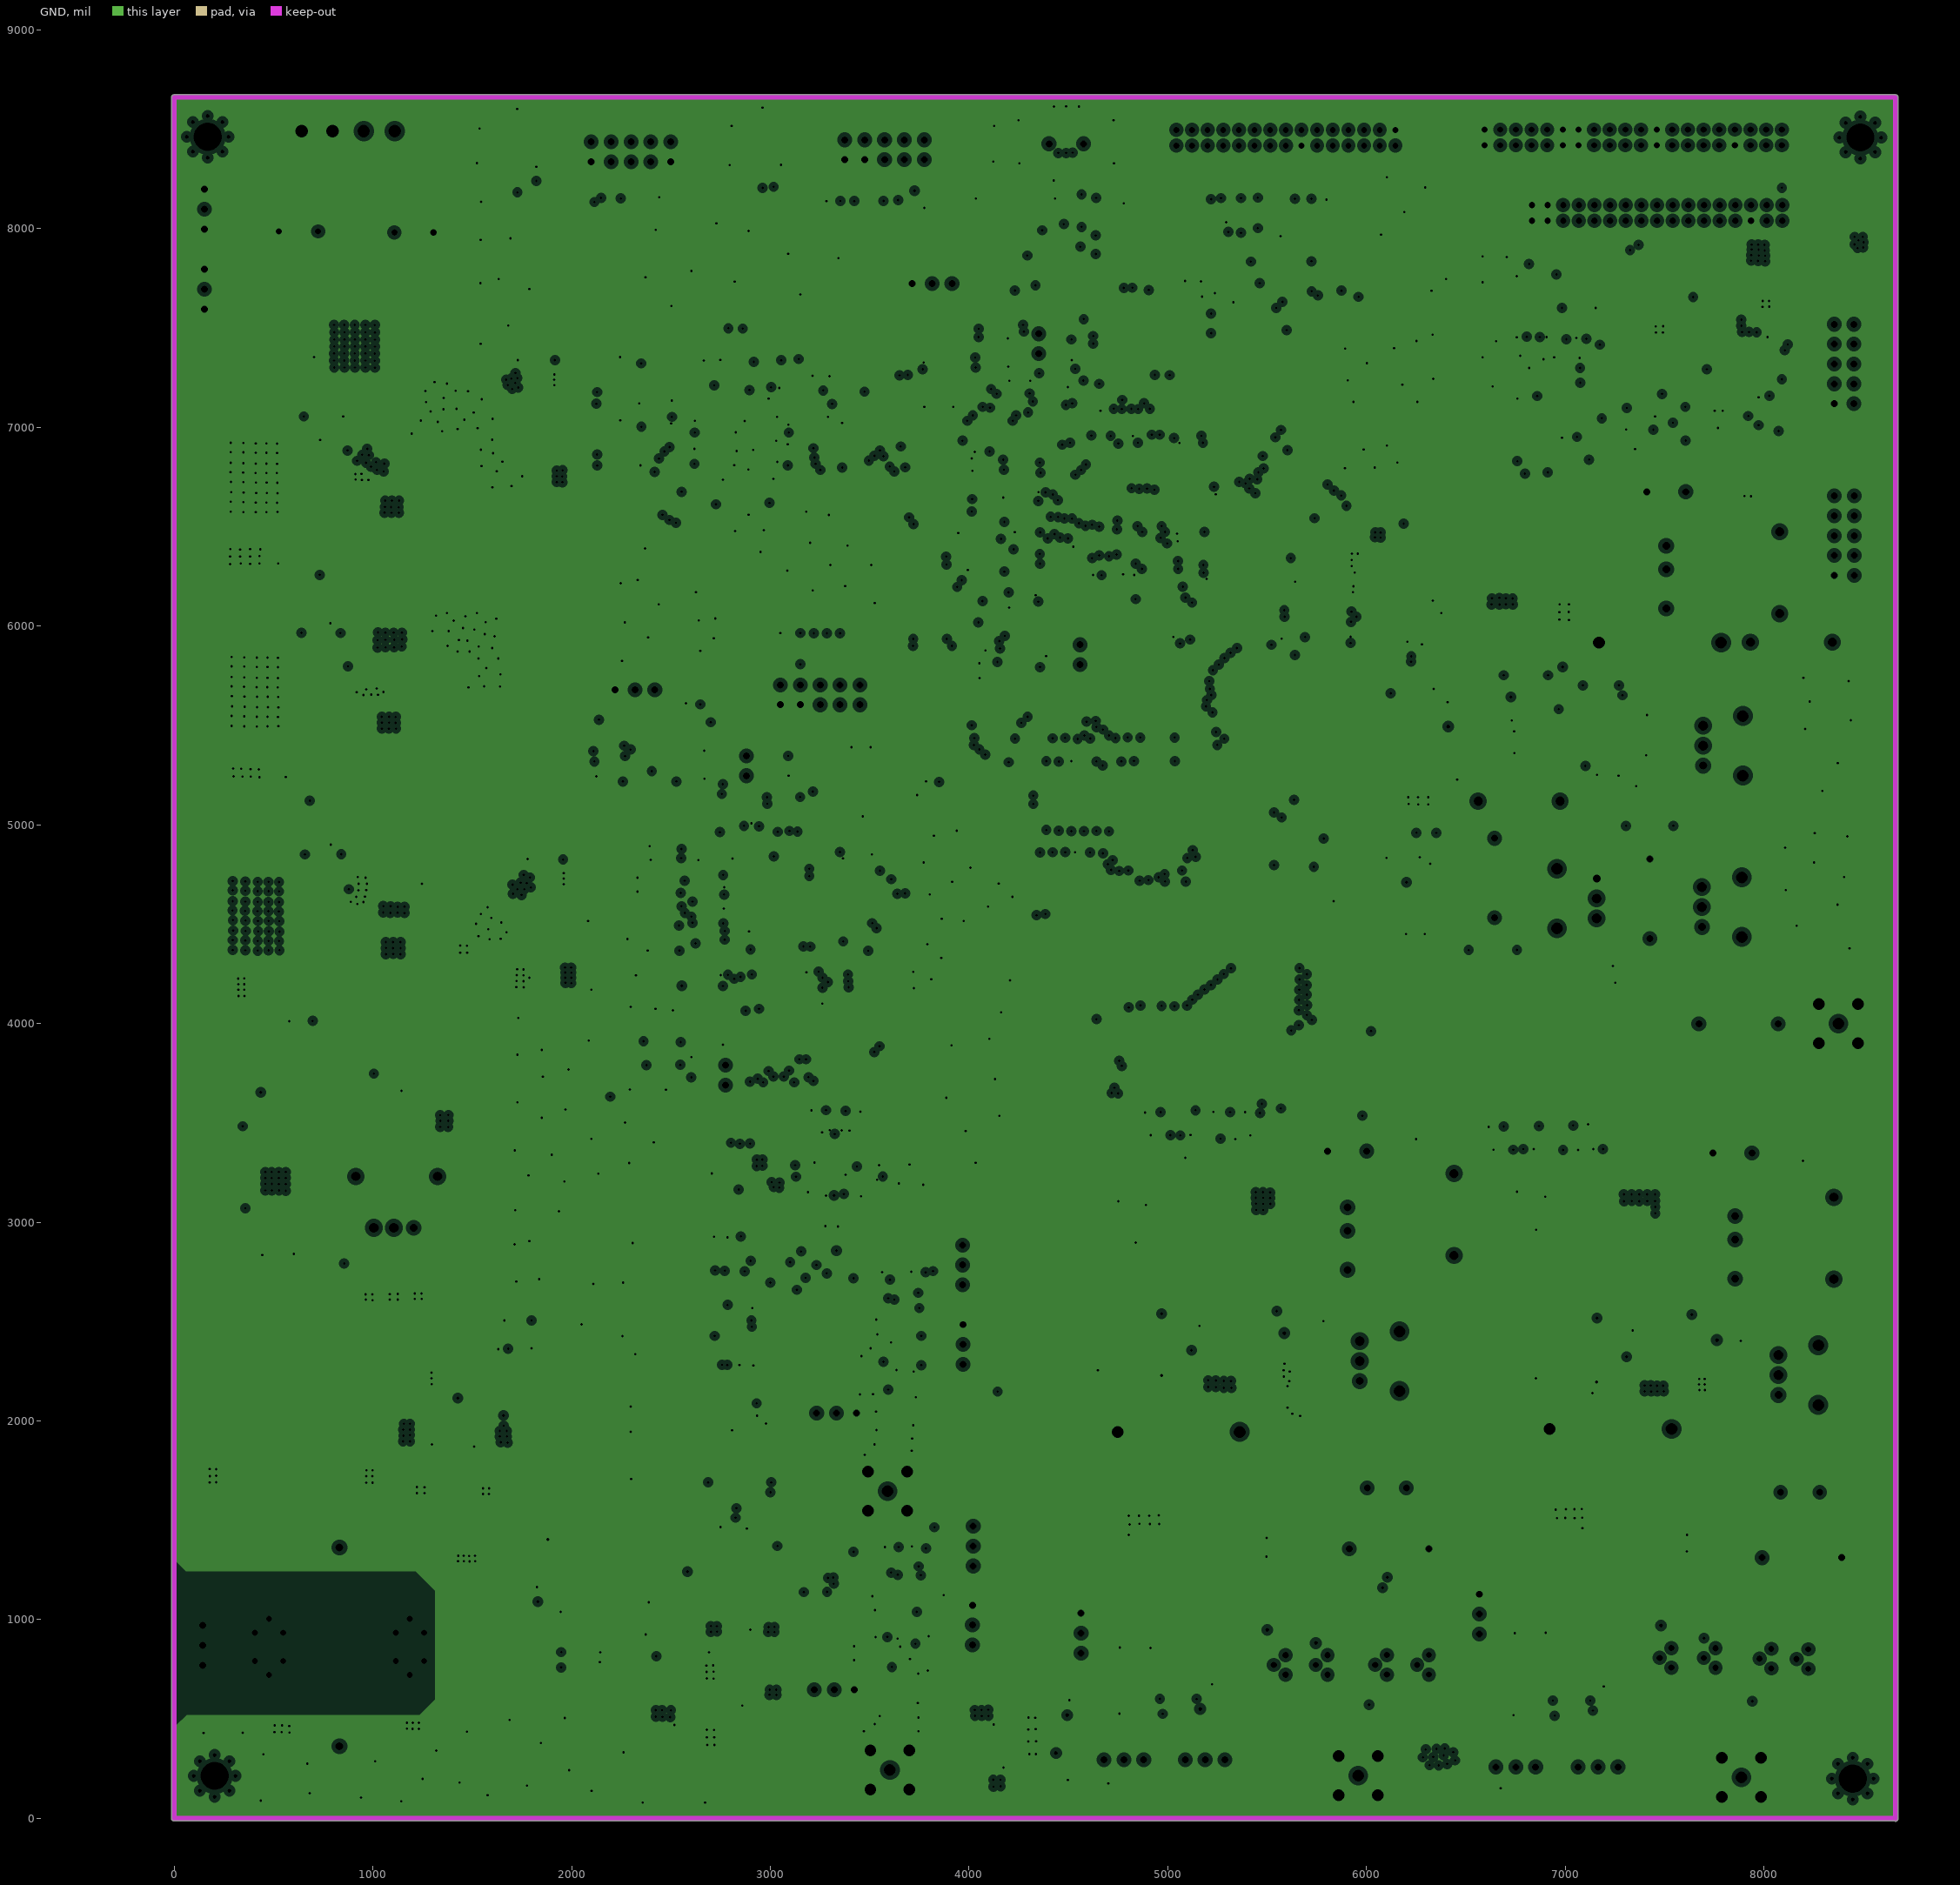
[diagram p0: GND, clearances drawn from the general rule]
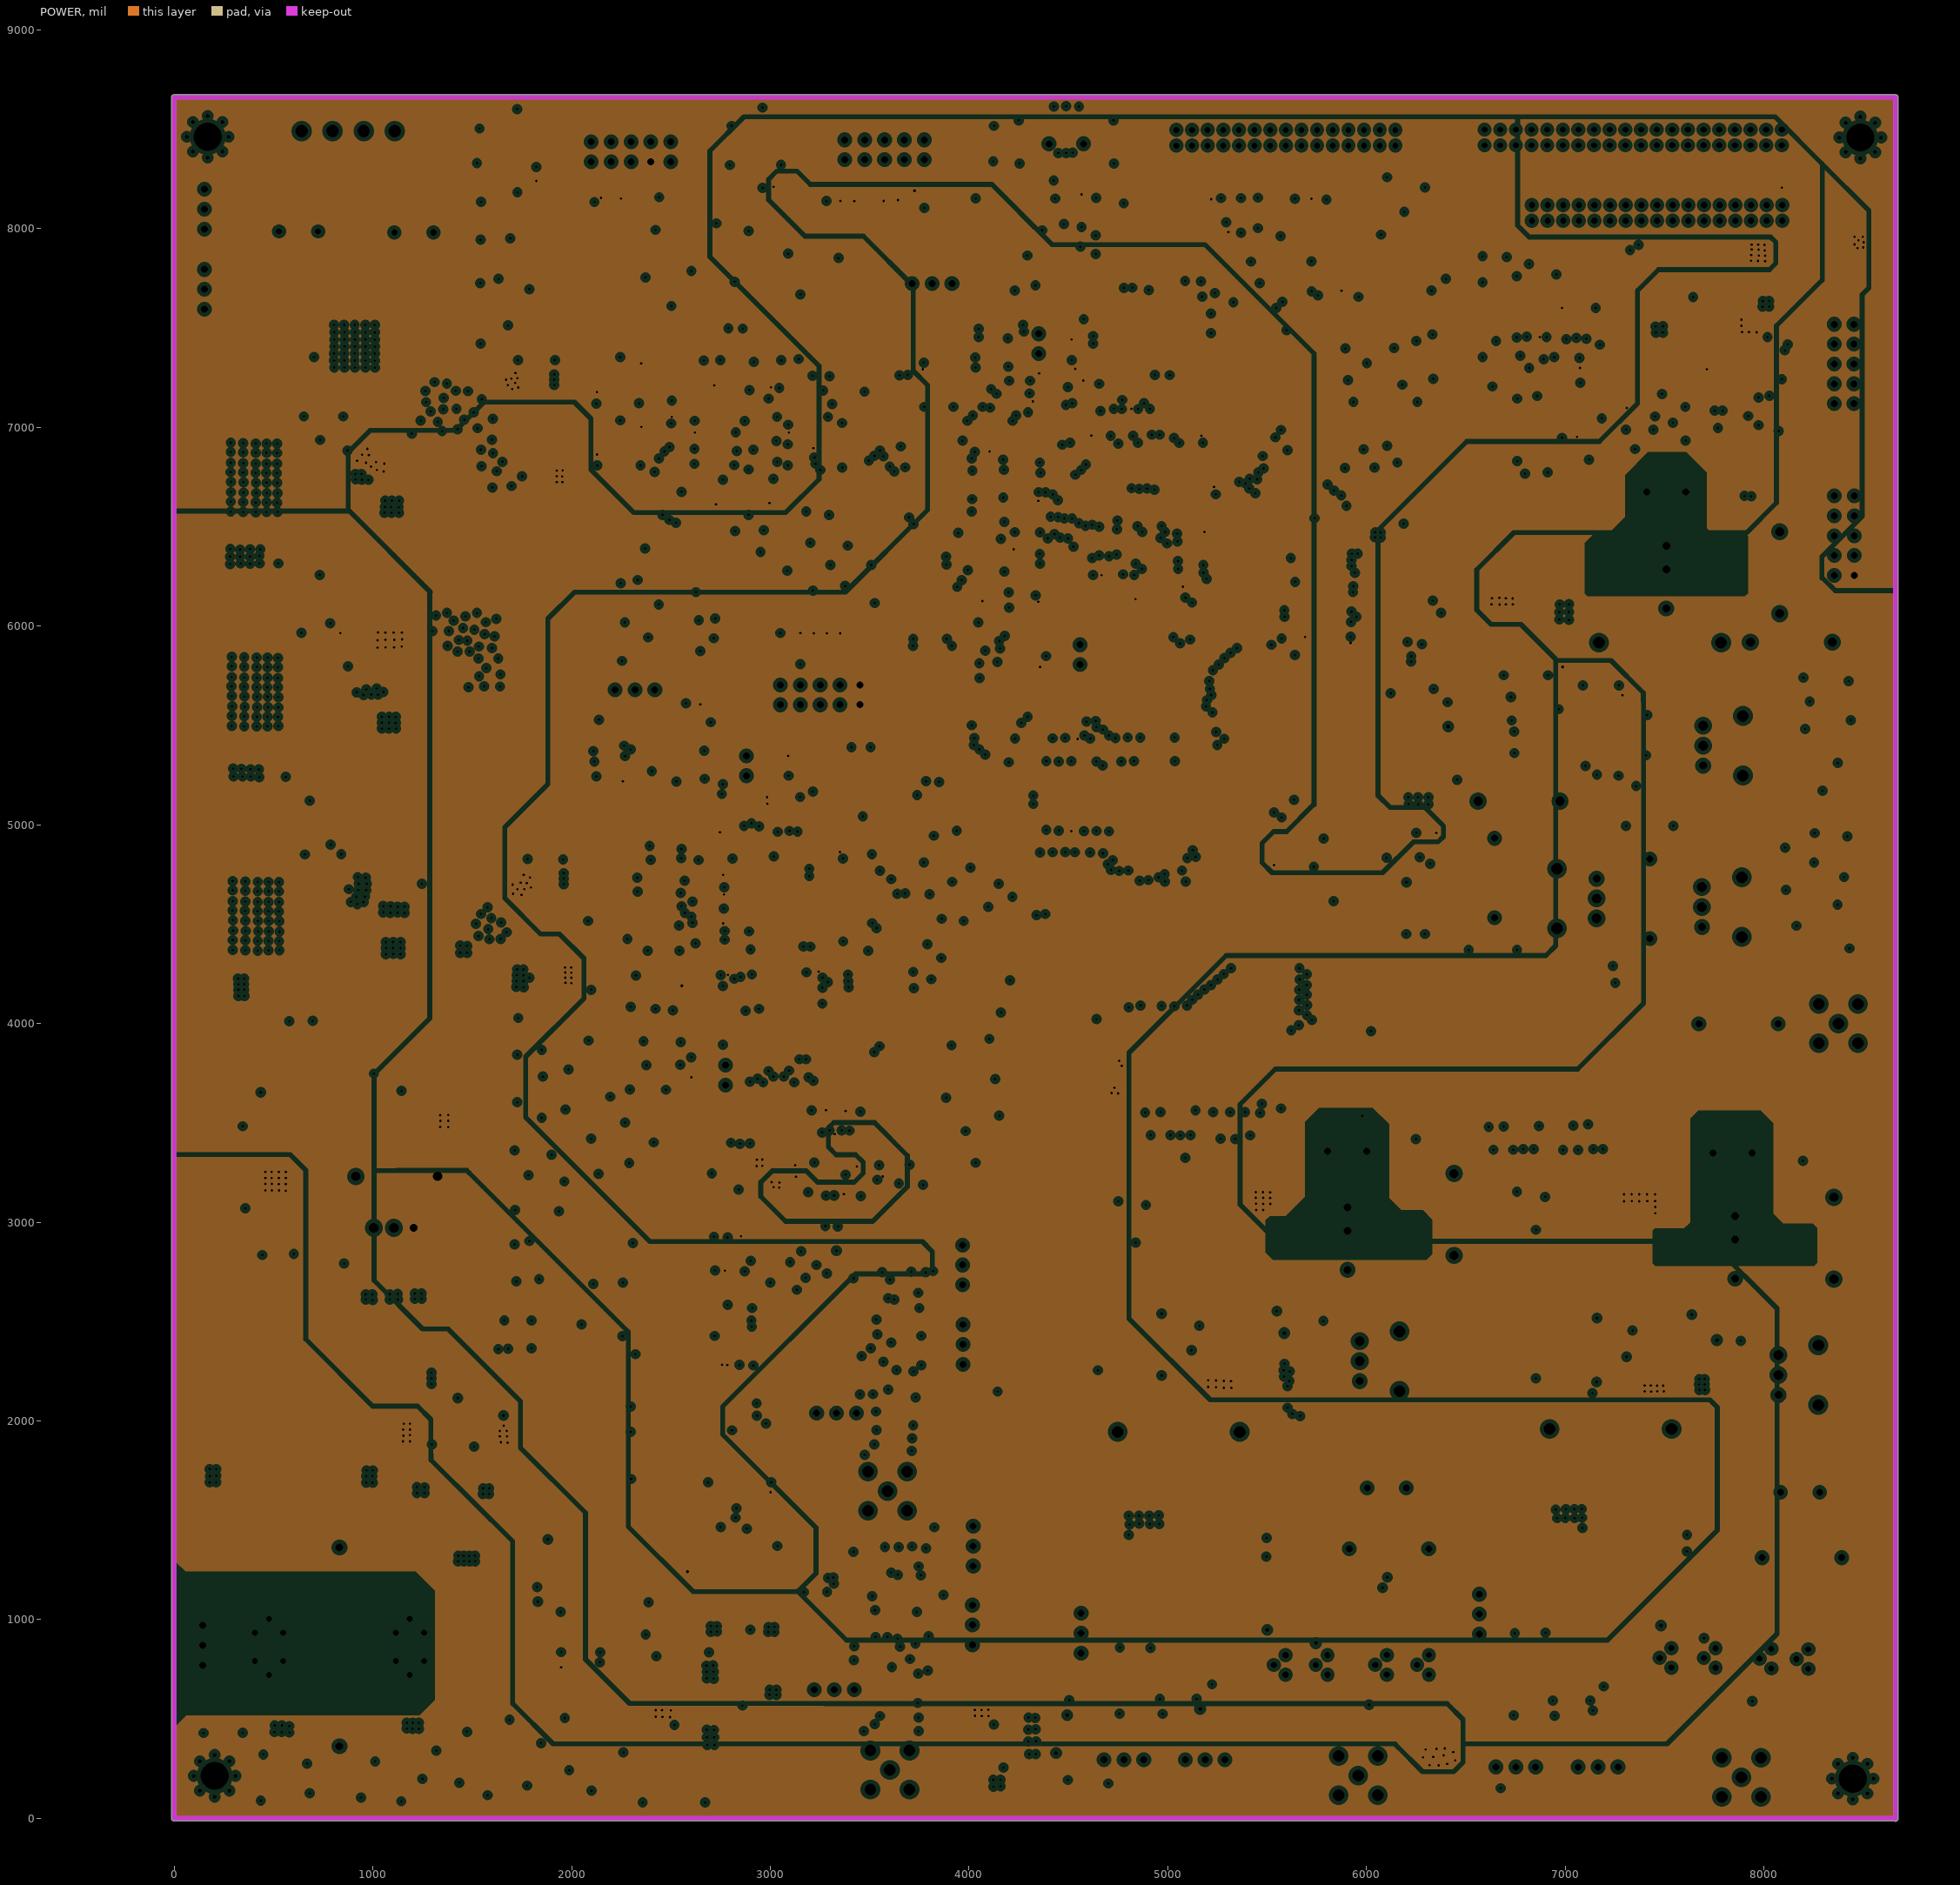
[diagram p1: POWER, clearances drawn from the general rule]
# Altium PCB MISC82309.PcbDoc (part 2 of 14)
## Components (designator, comment, footprint, x,y, rotation, side; value= is the part's Value field where it differs from the comment) (continued)
C229 "10uF/25V" CAP-ALU-5X5_4 1876,1836 r90 top
C230 "22uF/35V" CAP-ALU-6_3X5_4 1244,1946 r270 top
C231 "0.1uF" CAP_0805 1239,1919 r90 bottom
C232 "0.01uF" CAP_0603 2341,886 r180 top
C233 "0.1uF" CAP_0805 2086,799 r90 bottom
C240 "100pF" C0603 4465,8088 r270 bottom
C241 "1uF" C0603 4397,8088 r270 bottom
C242 "100nF" C0805 3545,5428 r90 bottom
C243 "100nF" C0805 3416,3509 r180 bottom
C244 "0.1uF" C0603 1755,8311 r180 bottom
C245 "100nF" C0805 2701,4612 r90 bottom
C246 "10uF" C0805 5266,3496 r0 bottom
C247 "10uF" C0805 3296,4838 r90 bottom
C248 "10uF" C0805 7935,7575 r270 bottom
C249 "10uF" C0805 3356,5428 r90 bottom
C250 "10uF" C0805 3488,3252 r90 bottom
C251 "10uF" C0805 2827,4293 r180 bottom
C252 "10uF" C0805 3196,4313 r0 bottom
C253 "10uF" C0805 3420,4836 r90 bottom
C254 "100nF" C0805 3245,3509 r0 bottom
C255 "100nF" C0805 3451,5428 r90 bottom
C256 "2.2uF" CAP_0805 3216,4138 r270 top
C257 "2.2uF" CAP_0805 3474,4807 r0 top
C263 "470pF" C1206 7823,2336 r0 bottom
C265 "47pF" C1206 7054,2328 r270 top
C266 "2.2uF/450V" CAP-EL-10X13_5-5 7841,3348 r0 top
C267 "22uF/35V" E6.3X5.4 7446,2256 r0 top
C270 "10nF" C1206 7248,2140 r180 bottom
C271 "2.2nF" C1206 7219,2455 r0 bottom
C276 "0.22nF" CAP_0805 7219,151 r180 bottom
C277 "0.1uF" CAP_0805 7514,1344 r0 top
C278 "0.47uF" C1206 6791,152 r180 bottom
C279 "0.33uF/400V" CBB-400V-10mm 8191,1312 r180 top
C280 "470pF" C0603 4811.5,3106 r0 top
C281 "470pF" C0603 6825,3154 r0 top
C282 "0.1uF" CAP_0805 6829,3425 r180 bottom
C283 "0.1uF" CAP_0805 7153,3425 r180 bottom
C284 "0.1uF" CAP_0805 6653,3424 r180 bottom
C285 "0.1uF" CAP_0805 7027,3318 r180 bottom
C288 "470pF" C0603 3595,2230 r270 bottom
C289 "1.5nF" C0603 3456,2228 r270 top
C290 "1.5nF" C0603 3782,2674 r270 top
C291 "0.01uF" C0603 3643,2542 r270 bottom
C292 "0.01uF" C0603 3612,2437 r180 bottom
C293 "0.22uF" C0603 3821,2505 r0 bottom
C311 "39pF" CAP_0603 2753,2546 r0 bottom
C317 "1uF" CAP_0805 6246,4488 r270 top
C318 "0.1uF" CAP_0805 6152,4488 r270 top
C330 "39pF" CAP_0603 2724,2664 r270 bottom
C363 "0.47uF" C0603 8002,6979 r0 bottom
C364 "330pF" C0603 7852,7062 r270 bottom
C370 "0.1uF" CAP_0603 7663,6966 r270 bottom
C373 "0.1uF" CAP_0805 6943,7263 r270 top
C374 "0.1uF" CAP_0805 7225,6989 r180 bottom
C411 "0.1uF" CAP_0603 3353,3408 r180 bottom
C412 "0.1uF" CAP_0603 3173,3265 r270 bottom
C413 "4.7uF" CAP_0603 3322,3183 r0 bottom
C420 "100nF" CAP_0603 2845,2208 r270 top
C421 "10uF" CAP_0603 2915,2208 r270 top
C422 "10uF" CAP_0603 2738,2041 r90 top
C423 "10uF" CAP_0603 2977,2058 r270 top
C424 "100nF" CAP_0603 2977,2058 r90 bottom
C449 "22uF" C0805 1826,7248 r180 top
C501 "39pF" CAP_0603 2878,1661 r270 bottom
C502 "39pF" CAP_0603 2814,1661 r270 bottom
C506 "Cap Semi" C0603 3277,3046 r270 top
C507 "Cap Semi" C0603 3340,3046 r270 top
C599 "0.1uF" CAP_0603 2717,2838 r90 top
CH-DET_A "SMB" SMB_V-RJ45#1 3602,243 r0 top
CH-DET_B "SMB" SMB_V-RJ45#1 3590,1646 r0 top
CHARGE-OUT_A "SMB" SMB_V-RJ45#2 5958,216 r90 top
CHARGE-OUT_B "SMB" SMB_V-RJ45#2 7887,207 r90 top
CPLD-JTAG "IDC2X5-2_54" IDC2X5-2_54 2499,8437 r180 top
CPLD_REST "SW" SW-6X3X2.5 1727,8394 r270 top
D2 "1N5822" D1810 1266,5393 r180 bottom
D3 "1N5822" D1810 1295,6476 r180 bottom
D4 "1N5822" D1810 1287,4257 r180 bottom
D5 "UF4007" "DO-41 - 10.46mm" 6440,3039 r90 top
D6 "SB560" SB560 4748,1945 r0 top
D10 "1N4004" "DO-41 - 10.46mm" 1120,3231 r180 top
D11 "ZPY15" "DO-41 - 10.46mm" 8138,5919 r180 top
D13 "UF4007" "DO-41 - 10.46mm" 8079,6269 r90 top
D14 "SB560" DO-201AD 7170,5917 r0 top
D15 "UF4007" "DO-41 - 10.46mm" 6768,5119 r0 top
D23 "1SMA4728A" DO-214AC 2762,3950 r90 top
D24 "4.7V" SOD-123 6859,7267 r270 top
D25 "1N4148WS" SOD323 3645,516 r180 top
D26 "1N4148WS" SOD323 3645,453 r0 top
D27 "1N4148" SOD-323 3691,1144 r0 bottom
D28 "1SMA4728A" DO-214AC 2281,4493 r0 top
D29 "1SMA4728A" DO-214AC 2293,3726 r90 top
D30 "50WQ03FN" TO-252AA 913,7478 r270 top
D31 "1N4148WS" SOD323 7513,6920 r0 top
D32 "1N4148WS" SOD323 1651,1089 r180 bottom
D33 "1N4148WS" SOD323 2107,1276 r180 top
D34 "1SMA4728A" DO-214AC 2475,3724 r90 top
D35 "SB560" SB560 6921,1960 r0 top
D38 "10BQ060" DO-214AA-L 1876,2195 r270 top
D40 "UF4007(US1M)" DO-214AA 7578,7579 r90 top
D41 "UF4007" "DO-41 - 10.46mm" 8351,2920 r90 top
D42 "1N4148" DO-213AA 7634,971 r180 top
D43 "1N4148" DO-213AA 7498,475 r0 top
D44 "1N4148" DO-213AA 8283,589 r0 top
D45 "1N4148" DO-213AA 7426,4998 r180 bottom
D46 "1N4148WS" SOD323 3632,1850 r0 top
D47 "1N4148WS" SOD323 3632,1912 r180 top
D48 "1N4148" SOD-323 3721,2525 r0 bottom
D49 "1N4148" DO-213AA 6642,4371 r180 bottom
D52 "4.7V" SOD-123 7246,6891 r180 top
D54 "4.7V" SOD-123 7041,7283 r270 bottom
D55 "IN4001/M1" DO-214AC 6260,5390 r270 top
D102 "1N4148" DO-213AA 5680,950 r180 top
D103 "1N4148" DO-213AA 5561,455 r0 top
D104 "1N4148" DO-213AA 6330,572 r0 top
D131 "1N4148WS" SOD323 8005,6913 r180 top
D-JTAG "IDC2X5-2_54" IDC2X5-2_54 3451,5704 r180 top
D_BOOT0 "PLS-2" PLS-2-2_54 2880,5347 r270 top
D_BOOT1 "PLS-2" PLS-2-2_54 2775,3690 r90 top
D_ISP "KF2510-3A" KF2510-3A 2319,5680 r0 top
D_REST "SW" SW-6X3X2.5 2648,5671 r90 top
ESD23 "PESD5V0S1BA" SOD323 4427,8542 r270 bottom
ESD24 "PESD5V0S1BA" SOD323 4553,8542 r270 bottom
ESD25 "PESD5V0S1BA" SOD323 4489,8542 r270 bottom
FAN1 "KF2510-3A" KF2510-3A 152,8098 r90 top
FAN2 "KF2510-3A" KF2510-3A 152,7695 r90 top
FB1 "60" SMD1206-L 2237,7322 r180 top
FB3 "60" SMD0805-L 6125,6013 r180 top
FB4 "60" SMD1206-L 2239,7003 r180 top
FB5 "60" SMD0805-L 4439,558 r270 top
FB6 "60" SMD0805-L 4438,228 r90 top
FB18 "60" SMD0805-L 7067,7511 r180 bottom
FB19 "60" SMD0805-L 2802,531 r270 top
FB20 "60" SMD0805-L 2801,857 r270 top
FB25 "60" SMD1206-L 8438,8137 r180 top
FB26 "60" SMD1206-L 8438,8024 r180 top
FB27 "60" SMD0805-L 2002,797 r270 bottom
FUSE1 "ASMD050-1812(30V,0.5A)" SMD1812-Fuse 5043,2788 r0 top
FUSE2 "ASMD050-1812(30V,0.5A)" SMD1812-Fuse 6506,6283 r0 top
FUSE12 "ASMD050-1812(30V,0.5A)" SMD1812-Fuse 7058,2787 r0 top
FUSE13 "ASMD050-1812(30V,0.5A)" SMD1812-Fuse 6835,6284 r180 top
FUSE14 "ASMD050-1812(30V,0.5A)" SMD1812-Fuse 5336,2989 r270 top
FUSE15 "ASMD050-1812(30V,0.5A)" SMD1812-Fuse 7334,2933 r270 top
GPIO&PWM "HEAD2X20-2MM-A" IDC2X20-2.0mm-A 6594,8420 r0 top
HV "KF2510-3A" KF2510-3A 144,871 r90 top
L2 "68uH" L330 1090,5298 r0 top
L3 "68uH" L330 1091,6394 r0 top
L4 "68uH" L330 1095,4162 r0 top
L5 "200uH" L200/1.4A 5904,2918 r90 top
L6 "200uH" L200/1.4A 7508,6246 r90 top
L11 "600R,100MHz" R0805 4029,6172 r0 bottom
L13 "330uH" PBS5022 608,2219 r180 top
L14 "600R,100MHz" R0805 2462,4280 r0 top
L15 "200uH" L200/1.4A 7854,2874 r90 top
L16 "330uH" L-9x12 8182,1641 r180 top
L21 "600R,100MHz" R0805 2984,3241 r180 top
L111 "330uH" L-9x12 6102,1663 r180 top
LED1 "LED" LED_0805 1876,4828 r180 top
LED2 "LED" LED_0805 749,5965 r0 top
LED3 "LED" LED_0805 753,7055 r0 top
LED4 "LED" LED_0805 750,4852 r180 top
LED5 "LED" LED_0805 612,7354 r0 top
LED6 "LED" LED_0805 1824,7338 r180 top
MOD-OUT "SMB" SMB_V-RJ45#1 8375,4000 r90 top
P21 "MiniUSB" MiniUSB-A 4489,8427 r270 top
P-JTAG "IDC2X5-2_54" IDC2X5-2_54 3775,8447 r180 top
P_BOOT0 "PLS-2" PLS-2-2_54 4350,7471 r270 top
P_BOOT1 "PLS-2" PLS-2-2_54 4559,5806 r90 top
P_ISP "KF2510-3A" KF2510-3A 3814,7723 r0 top
P_REST "SW" SW-6X3X2.5 2961.17,8408 r90 top
PCB_MH1 "MOUNTING HOLE 3MM" MOUNTING_HOLE_3MM 8446,200 r90 top
PCB_MH2 "MOUNTING HOLE 3MM" MOUNTING_HOLE_3MM 8485,8459 r90 top
PCB_MH3 "MOUNTING HOLE 3MM" MOUNTING_HOLE_3MM 169,8462 r90 top
PCB_MH4 "MOUNTING HOLE 3MM" MOUNTING_HOLE_3MM 204,214 r90 top
POWER "HEAD4-3.96A" VH-3_96-4 642,8490 r0 top
Q1 "S9013LT1" SOT-23 444,2718 r180 top
Q3 "S9012LT1" SOT-23 1005,3699 r0 top
Q4 "IRF740" TO220V1 5966,2301 r0 top
Q7 "NPN/SS8050LT1" SOT-23-3 4684,8090 r180 top
Q8 "SI2301CDS-T1-GE3" SOT-23 4566,8052 r180 top
Q9 "IRF740" TO220V1 8073,2231 r0 top
Q10 "SI4435DY" SO-8_N 651,2999 r0 top
Q16 "IRF740" TO220V1 7694,5398 r0 top
Q19 "NPN/CJ2302" SOT-23-3 3647,692 r180 top
Q20 "NPN/CJ2302" SOT-23-3 3638,2082 r180 top
Q22 "IRF740S" D2PAK_N 1582,948 r270 top
Q25 "2SA1416" SOT89 7770,7581 r90 top
Q26 "MMBF170" SOT-23 8018,7334 r180 top
R1 "270R" RES_0805 1875,4825 r0 bottom
R2 "1K" RES_0805 750,5965 r180 bottom
R3 "470R" RES_0805 754,7055 r180 bottom
R4 "1K" RES_0805 750,4852 r180 bottom
R5 "100R" RES_0805 1043,3524 r180 top
R6 "47K" RES_0805 345,3572 r90 top
R7 "47K" RES_0805 396,3024 r0 top
R8 "1K" RES_0805 799,2755 r270 top
R9 "20K" RES_0805 613,7439 r0 top
R11 "47K" RES_0805 437,3572 r270 top
R12 "2.2K" RES_0805 565,2714 r180 top
R13 "2.2K" RES_0805 565,2798 r0 top
R15 "100K" RES_0805 1106,3749 r0 bottom
R16 "270R" RES_0805 1826,7338 r0 bottom
R17 "1K8" R1206 4648,2367 r90 top
R18 "150K" R1206 5427,2554 r0 top
R19 "56K" R1206 5479,2494 r270 bottom
R22 "50R" RES_0805 4759,941 r270 top
R23 "22R" R1206 5722,2342 r90 top
R25 "1K" R1206 5723,2322 r0 bottom
R26 "8K2" R1206 5057,2289 r180 bottom
R27 "510R" RES_0805 4809,564 r90 bottom
R28 "4R7" R1206 5726,2078 r0 bottom
R29 "2R2" R1206 5725,2201 r0 bottom
R30 "20R" RES_0805 4837,941 r270 top
R31 "2.7K" RES_0805 4899,563 r270 bottom
R32 "100R" RES_0805 4799,803 r0 top
R33 "50R" RES_0805 4914,941 r90 top
R34 "2K" RES_0805 5051,3377 r0 bottom
R35 "0R" RES_0603 5874,7756 r270 top
R36 "0R" RES_0603 5336,7945 r180 bottom
R38 "1M" R1206 4860,2366 r90 top
R39 "1M" R1206 6249,3305 r270 bottom
R40 "1K5" R1206 5794,572 r0 top
R41 "1K5" R1206 6119,572 r0 top
R42 "390R" R1206 6332,456 r0 top
R43 "1K" R1206 6092,1003 r90 bottom
R44 "470R" RES_0805 5162,1170 r0 top
R45 "2K7" RES_0805 5408,1509 r180 top
R46 "2K7" RES_0805 5408,1411 r0 top
R47 "50R" RES_0805 5086,564 r90 bottom
R48 "3K3" RES_0805 5223,589 r270 top
R57 "0R" RES_0603 4394,8088 r270 top
R58 "10K" R0603 2187,7150 r90 bottom
R59 "22R" R0603 2386,7178 r90 top
R61 "10K" RES_0603 3020,5247 r0 top
R62 "10K" RES_0603 2634,3791 r180 top
R63 "10K" R0603 2989,8253 r180 bottom
R64 "10K" RES_0603 4485,7375 r0 top
R65 "10K" RES_0603 4424,5895 r180 top
R66 "1M" R0603 4111,6440 r270 bottom
R67 "10K" R0603 6306,6016 r180 top
R68 "10K" R0603 6306,6091 r180 top
R70 "20K" R1206 6574,5753 r0 top
R71 "1M" R1206 6571,5343 r90 top
R72 "10K" R1206 6233,5574 r90 top
R73 "20K" R1206 6681,5343 r90 top
R74 "1M" R1206 7918,6535 r270 bottom
R75 "8K2" R1206 7049,5363 r90 top
R76 "22K" R1206 6855,5470 r0 top
R77 "150K" R1206 7029,5640 r90 bottom
R78 "22K" R1206 6856,5580 r0 top
R79 "20K" R1206 6456,5342 r90 top
R80 "20K" R1206 6854,5686 r180 top
R81 "22R" R1206 7486,5550 r270 top
R82 "1K" R1206 7372,5360 r270 top
R84 "2R2" R1206 7467,5195 r0 bottom
R85 "2R2" R1206 7467,5300 r0 bottom
R87 "220R" R1206 7422,4996 r180 top
R89 "100R" RES_2512 7430,4125 r270 top
R91 "10R" RES_0805 6124,5836 r0 top
R92 "220R" R1206 6638,4371 r180 top
R95 "0R" RES_0603 4330,8088 r270 top
R96 "0R" RES_0603 4266,8088 r270 top
R98 "22R" R1206 7877,2270 r90 top
R100 "10K" R0603 1755,8240 r180 bottom
R101 "0R/NC" RES_0603 5258,8229 r90 top
R102 "0R/NC" RES_0603 5369,8228 r90 top
R103 "0R/NC" RES_0603 5452,8227 r90 top
R104 "0R/NC" RES_0603 5640,8225 r90 bottom
R106 "1K" R1206 2762,4075 r90 bottom
R108 "10K" R0603 2191,6836 r90 bottom
R109 "22R" R0603 2392,6869 r90 top
R110 "1K" R1206 2476,3851 r90 bottom
R111 "4.7K" R0603 2943,5078 r270 top
R112 "4.7K" R0603 2868,5078 r270 top
R113 "10K" R0603 2648,5544 r270 bottom
R114 "1M" R0603 2491,4691 r270 bottom
R149 "4.7K" R0603 4701,7966 r0 top
R150 "47K" RES_0603 4535,8088 r90 bottom
R151 "10K" R0603 4811.5,2938 r180 top
R152 "100R" R1206 6117,456 r0 top
R153 "12K" R1206 5911,947 r180 bottom
R154 "12K" R1206 5910,1058 r0 bottom
R155 "0R/NC" R0805 6846,7605 r180 bottom
R156 "0R" R0805 6846,7512 r0 bottom
R157 "4R7" R1206 7822,2020 r0 bottom
R158 "2R2" R1206 7822,2129 r0 bottom
R159 "1K" R1206 7822,2235 r0 bottom
R160 "8K2" R1206 7247,2263 r180 bottom
R161 "12K" R1206 5685,1057 r0 bottom
R162 "12K" R1206 5685,948 r180 bottom
R163 "150K" R1206 5685,572 r180 bottom
R164 "1.8K" R1206 5902,573 r180 bottom
R165 "10K" R0805 7030,7262 r90 top
R166 "680R" R0805 6774,7263 r270 bottom
R168 "1K" R0805 6859,7262 r270 bottom
R172 "330K" R0603 7515,7122 r180 top
R173 "1M" R0603 7515,7055 r180 top
R174 "330K" R0603 7515,7055 r180 bottom
R175 "0ohm" R0603 7515,6988 r0 top
R186 "10K" RES_0603 3614,836 r90 top